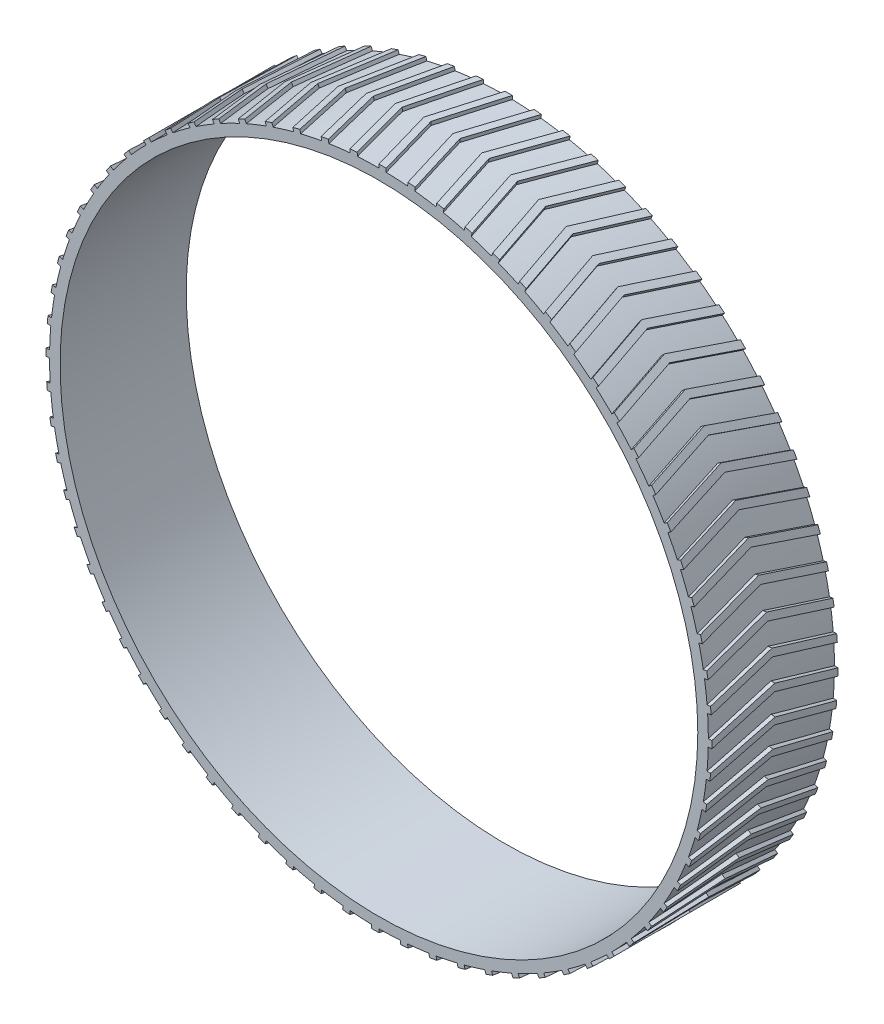
SolidWorks part; units mm, degrees
ref_plane "Front Plane" through (0, 0, 0) normal (0, 0, 1) x (1, 0, 0)
ref_plane "Top Plane" through (0, 0, 0) normal (0, 1, 0) x (1, 0, 0)
ref_plane "Right Plane" through (0, 0, 0) normal (1, 0, 0) x (0, 0, -1)
sketch "Sketch1" plane through (0, 0, 0) normal (0, 0, 1) x (1, 0, 0)
  circle A0 centre (0, 0) radius 94
  circle A1 centre (0, 0) radius 91
  dimension "D1" = 188
  dimension "D2" = 182
extrude "Boss-Extrude1" add sketch "Sketch1" along normal blind 36
sketch "Sketch3" plane through (0, 0, 0) normal (0, 1, 0) x (1, 0, 0)
  line L0 (0, 0) -> (-5.1929, -18)
  line L1 (-5.1929, -18) -> (0, -36)
  line L2 (-94, -36) -> (94, -36) construction
  line L3 (2.0816, 0) -> (-3.1113, -18)
  line L4 (-3.1113, -18) -> (2.0816, -36)
  line L5 (0, 0) -> (2.0816, 0)
  line L8 (0, -36) -> (2.0816, -36)
  line L9 (-3.1113, -18) -> (1.9216, -35.4456) construction
  line L10 (1.9216, -0.5544) -> (-3.1113, -18) construction
  dimension "D1" = 2
extrude "Boss-Extrude2" add sketch "Sketch3" along normal blind 3 from offset 92
pattern_circular "CirPattern1" count 72 over 360 about axis through (0, 0, 0) along (0, 0, 1) of "Boss-Extrude2"
